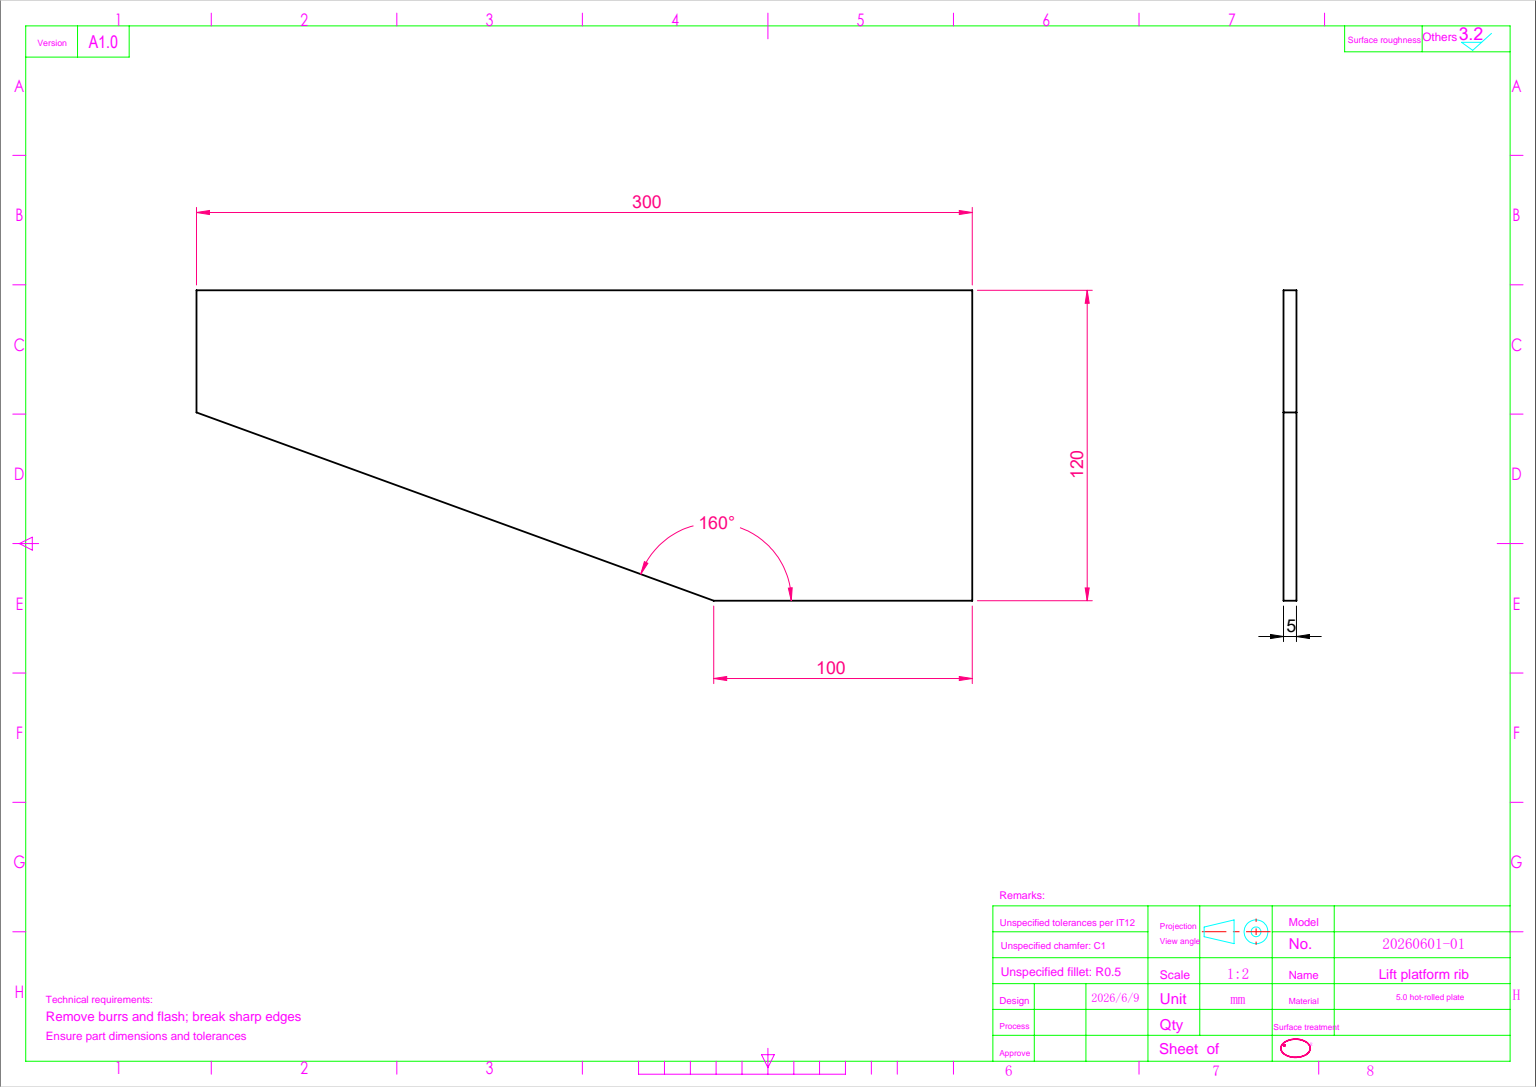
SolidWorks part; units mm, degrees
ref_plane "前视基准面" through (0, 0, 0) normal (0, 0, 1) x (1, 0, 0)
ref_plane "上视基准面" through (0, 0, 0) normal (0, 1, 0) x (1, 0, 0)
ref_plane "右视基准面" through (0, 0, 0) normal (1, 0, 0) x (0, 0, -1)
sketch "草图1" plane through (0, 0, 0) normal (0, 0, 1) x (1, 0, 0)
  line L0 (0, 0) -> (300, 0)
  line L1 (300, 0) -> (300, -120)
  line L2 (300, -120) -> (200, -120)
  line L3 (200, -120) -> (0, -47.206)
  line L4 (0, -47.206) -> (0, 0)
  dimension "D1" = 300
  dimension "D2" = 120
  dimension "D3" = 100
  dimension "D4" = 160
extrude "凸台-拉伸1" add sketch "草图1" along normal blind 5
